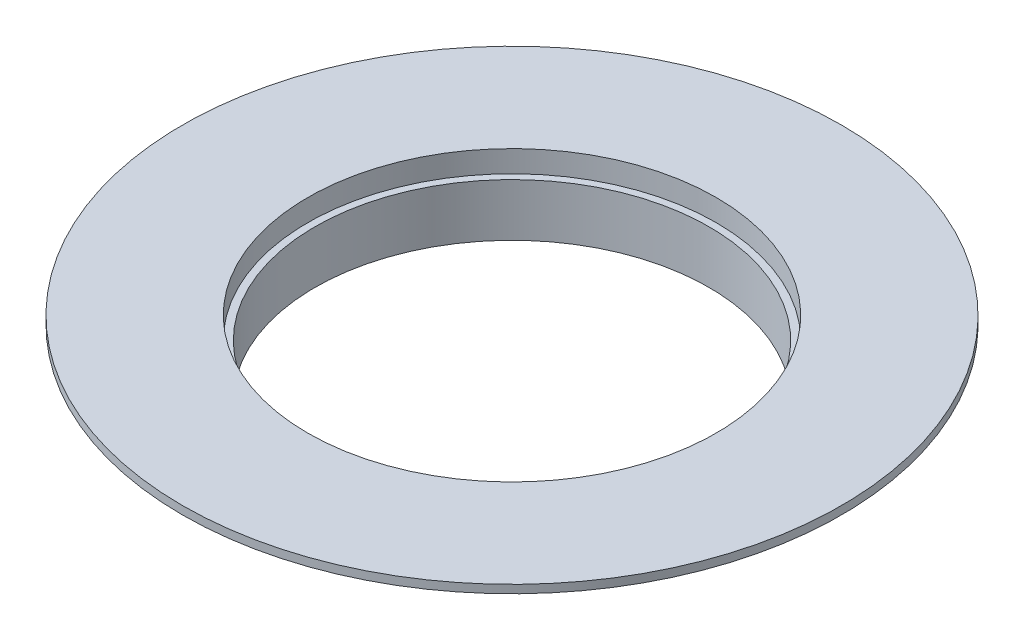
from build123d import *


with BuildPart() as part:
    # Sketch1 → Revolve1 (revolve)
    with BuildSketch(Plane.XY, mode=Mode.PRIVATE) as revolve1_sk:
        Polygon((102, 158), (65.583048881, 158), (65.583048881, 151.5), (63.995706961, 151.5), (63.995706961, 137.5), (60.995706961, 137.5), (60.995706961, 153.778962031), (63.193534924, 153.778962031), (63.193534924, 160.531936258), (102, 160.531936258), align=None)
    revolve(revolve1_sk.sketch.rotate(Axis((0, 0, 0), (0, -1, 0)), 90), axis=Axis((0, 0, 0), (0, -1, 0)))


solid = part.part
